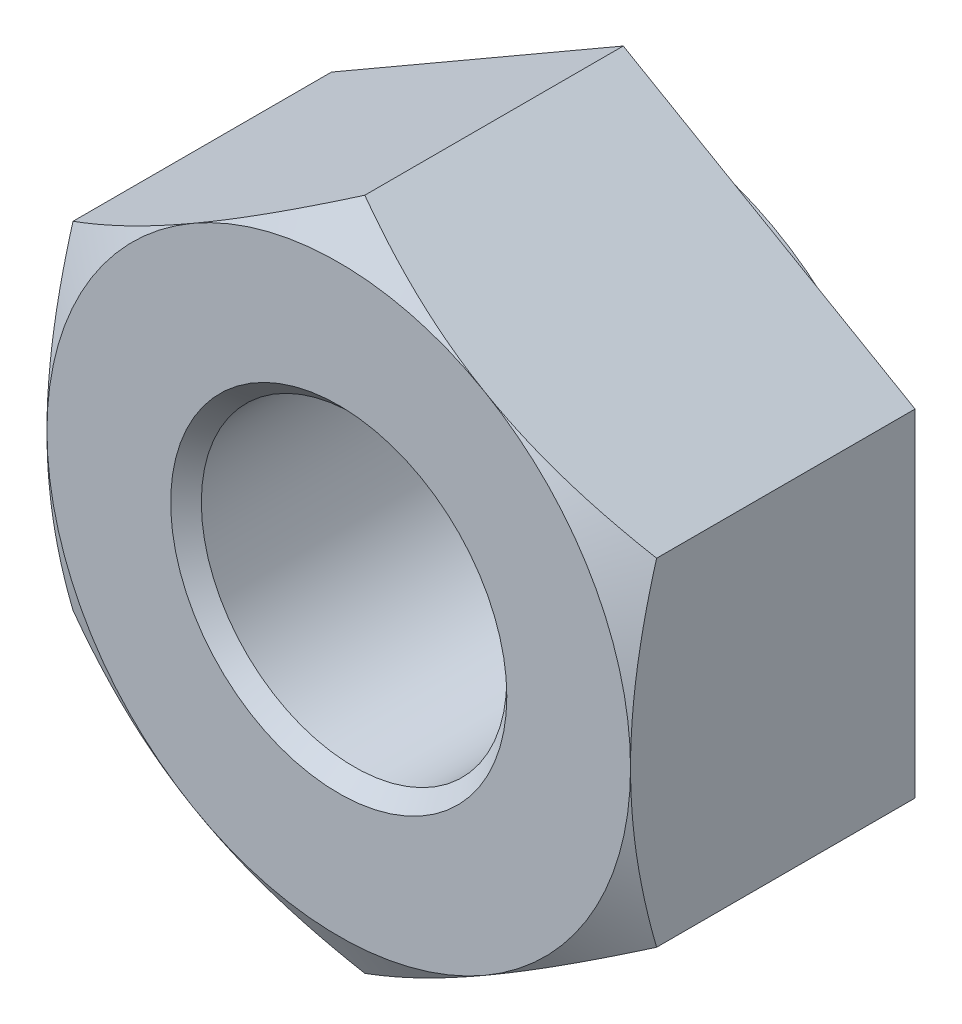
SolidWorks part; units mm, degrees
material "钢"
ref_plane "Front Plane" through (0, 0, 0) normal (0, 0, 1) x (1, 0, 0)
ref_plane "Top Plane" through (0, 0, 0) normal (0, 1, 0) x (1, 0, 0)
ref_plane "Right Plane" through (0, 0, 0) normal (1, 0, 0) x (0, 0, -1)
sketch "Dimension sketch" plane through (0, 0, 0) normal (0, 0, 1) x (1, 0, 0)
  line L0 (0, 0) -> (10, 0) construction
  point P3 (10.8, 0)
  point P4 (1.5, 0)
  point P5 (0.6, 0)
  point P6 (14.6, 0)
  point P7 (17.77, 0)
  point P8 (8.4, 0)
  point P9 (6.43, 0)
  point P10 (16, 0)
  dimension "D" = 10
  dimension "da(最大)" = 10.8
  dimension "P" = 1.5
  dimension "c(最大)" = 0.6
  dimension "dw(最小)" = 14.6
  dimension "e(最小)" = 17.77
  dimension "m(最大)" = 8.4
  dimension "m´(最小)" = 6.43
  dimension "s(最大)" = 16
sketch "Sketch1" plane through (0, 0, 0) normal (0, 0, 1) x (1, 0, 0)
  line L1 (0, 9.2376) -> (-8, 4.6188)
  line L2 (-8, 4.6188) -> (-8, -4.6188)
  line L3 (-8, -4.6188) -> (0, -9.2376)
  line L4 (0, -9.2376) -> (8, -4.6188)
  line L5 (8, -4.6188) -> (8, 4.6188)
  line L6 (8, 4.6188) -> (0, 9.2376)
  circle A0 centre (0, 0) radius 8 construction
  circle A1 centre (0, 0) radius 4.1881
  dimension "dm" = 8.3763
  dimension "s" = 16
extrude "Extrude1" add sketch "Sketch1" along normal blind 8.4
cosmetic thread "Cosmetic Thread1" parameters "D2"=10
sketch "Sketch2" plane through (0, 0, 0) normal (0, 0, 1) x (1, 0, 0)
  circle A0 centre (0, 0) radius 7.3
  dimension "dw" = 14.6
extrude "Cut-Extrude2" cut sketch "Sketch2" along normal blind 0.6 flip side to cut
sketch "Sketch3" plane through (0, 0, 8.4) normal (0, 0, 1) x (1, 0, 0)
  line L0 (0, -9.2376) -> (8, -4.6188) construction
  circle A0 centre (0, 0) radius 8
extrude "Cut-Extrude3" cut sketch "Sketch3" against normal through all draft 60 flip side to cut
chamfer "Chamfer1" distance 0.42 angle 45 2 edges at (4.1881, 0, 0) (4.1881, 0, 8.4)
